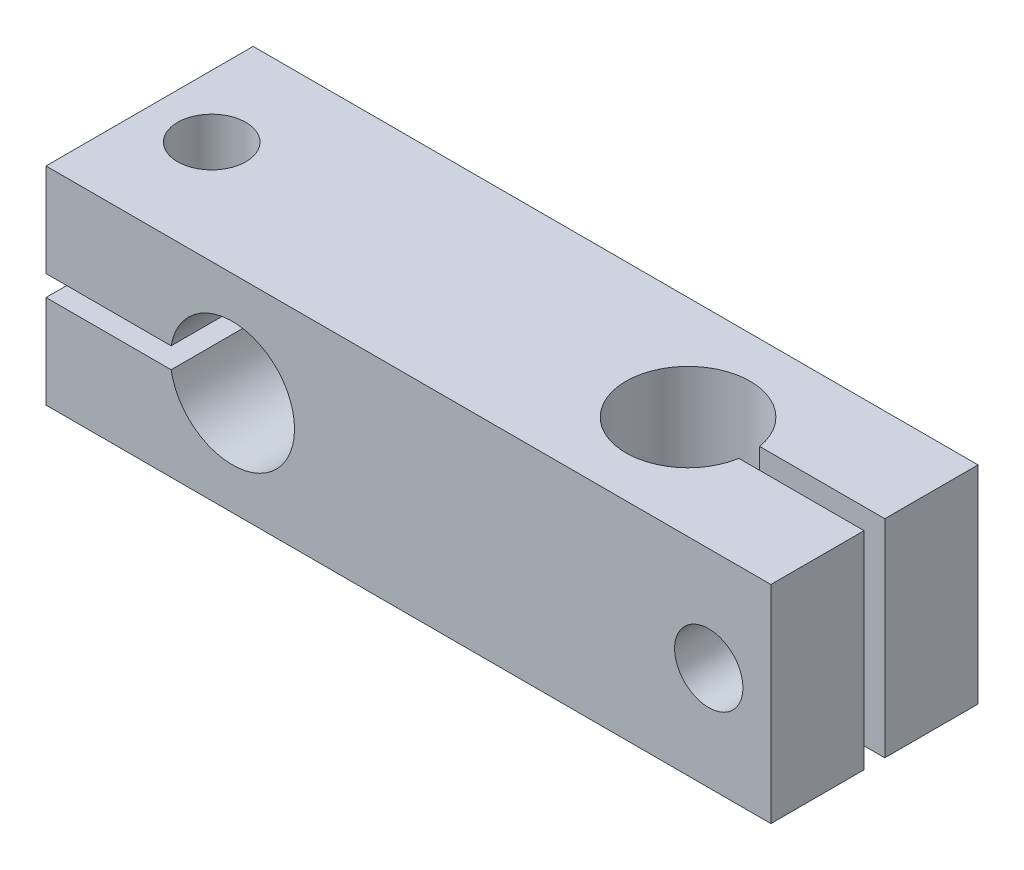
from build123d import *

# Parameters (mm, degrees)
SKETCH1_R             = 2
BOSS_EXTRUDE1_DEPTH   = 20
HOLE1_D               = 6.6
HOLE1_DEPTH           = 9
M6_TAPPED_HOLE1_D     = 5
M6_TAPPED_HOLE1_DEPTH = 9
M6_TAPPED_HOLE1_TIP   = 1.502151548
SKETCH6_R             = 2
CUT_EXTRUDE1_DEPTH    = 51.206971578
M6_TAPPED_HOLE2_D     = 5
M6_TAPPED_HOLE2_DEPTH = 9
M6_TAPPED_HOLE2_TIP   = 1.502151548
HOLE2_D               = 6.6
HOLE2_DEPTH           = 9


with BuildPart() as part:
    # Sketch1 → Boss-Extrude1 (new body)
    with BuildSketch(Plane.XY):
        with BuildLine():
            Line((-41.48180318, 24.678559646), (28.51819682, 24.678559646))
            Line((28.51819682, 24.678559646), (28.51819682, 4.678559646))
            Line((28.51819682, 4.678559646), (-41.48180318, 4.678559646))
            Line((-41.48180318, 4.678559646), (-41.48180318, 13.678559646))
            Line((-41.48180318, 13.678559646), (-29.397882963, 13.678559646))
            ThreePointArc((-29.397882963, 13.678559646), (-17.48180318, 14.678559646), (-29.397882963, 15.678559646))
            Line((-29.397882963, 15.678559646), (-41.48180318, 15.678559646))
            Line((-41.48180318, 15.678559646), (-41.48180318, 24.678559646))
        make_face()
        with Locations((22.51819682, 14.678559646)):
            Circle(SKETCH1_R, mode=Mode.SUBTRACT)
    extrude(amount=BOSS_EXTRUDE1_DEPTH)

    # Hole1
    with Locations(Plane.XY.offset(20)):
        with Locations((22.51819682, 14.678559646)):
            Hole(HOLE1_D / 2, depth=HOLE1_DEPTH)

    # M6 Tapped Hole1
    with Locations(Plane(origin=(0, 0, 0), x_dir=(-1, 0, 0), z_dir=(0, 0, -1))):
        with Locations((-22.51819682, 14.678559646)):
            Hole(M6_TAPPED_HOLE1_D / 2, depth=M6_TAPPED_HOLE1_DEPTH)
            with Locations((0, 0, -(M6_TAPPED_HOLE1_DEPTH + M6_TAPPED_HOLE1_TIP / 2))):  # 118° drill point
                Cone(0, M6_TAPPED_HOLE1_D / 2, M6_TAPPED_HOLE1_TIP, mode=Mode.SUBTRACT)

    # Sketch6 → Cut-Extrude1 (cut, through all)
    with BuildSketch(Plane(origin=(0, 24.678559646, 0), x_dir=(1, 0, 0), z_dir=(0, 1, 0))):
        with Locations(Location((-35.48180318, -10, 0), (0, 0, 270))):
            Circle(SKETCH6_R)
        with BuildLine():
            Line((16.434276603, -11), (30.650689968, -11))
            Line((30.650689968, -11), (30.650689968, -9))
            Line((30.650689968, -9), (16.434276603, -9))
            ThreePointArc((16.434276603, -9), (4.51819682, -10), (16.434276603, -11))
        make_face()
    extrude(amount=-CUT_EXTRUDE1_DEPTH, mode=Mode.SUBTRACT)

    # M6 Tapped Hole2
    with Locations(Plane(origin=(0, 4.678559646, 0), x_dir=(-1, 0, 0), z_dir=(0, -1, 0))):
        with Locations((35.48180318, -10)):
            Hole(M6_TAPPED_HOLE2_D / 2, depth=M6_TAPPED_HOLE2_DEPTH)
            with Locations((0, 0, -(M6_TAPPED_HOLE2_DEPTH + M6_TAPPED_HOLE2_TIP / 2))):  # 118° drill point
                Cone(0, M6_TAPPED_HOLE2_D / 2, M6_TAPPED_HOLE2_TIP, mode=Mode.SUBTRACT)

    # Hole2
    with Locations(Plane(origin=(0, 24.678559646, 0), x_dir=(1, 0, 0), z_dir=(0, 1, 0))):
        with Locations((-35.48180318, -10)):
            Hole(HOLE2_D / 2, depth=HOLE2_DEPTH)


solid = part.part
